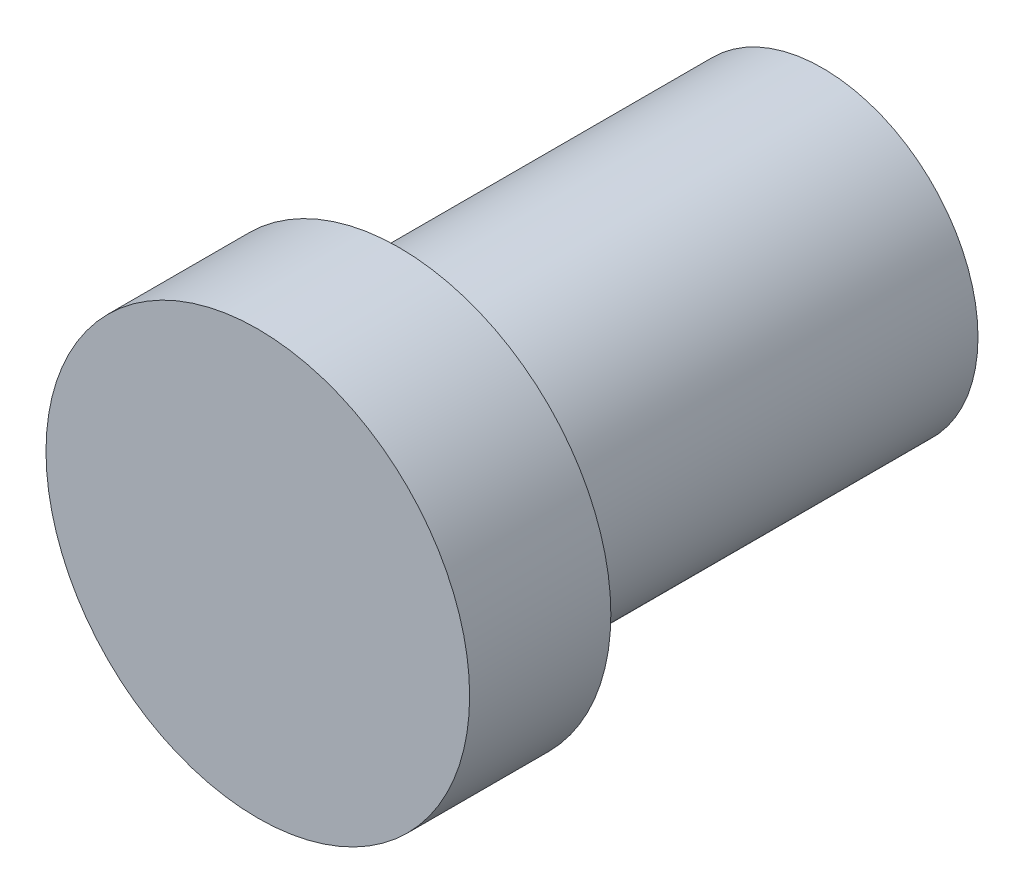
from build123d import *

# Parameters (mm, degrees)
SKETCH_1_R      = 2.2
EXTRUDE_1_DEPTH = 6
SKETCH_2_R      = 3
EXTRUDE_2_DEPTH = 2


with BuildPart() as part:
    # 草图1 → 凸台-拉伸1 (new body)
    with BuildSketch(Plane.XY):
        Circle(SKETCH_1_R)
    extrude(amount=-EXTRUDE_1_DEPTH)

    # 草图2 → 凸台-拉伸2 (add)
    with BuildSketch(Plane.XY):
        Circle(SKETCH_2_R)
    extrude(amount=EXTRUDE_2_DEPTH)


solid = part.part
